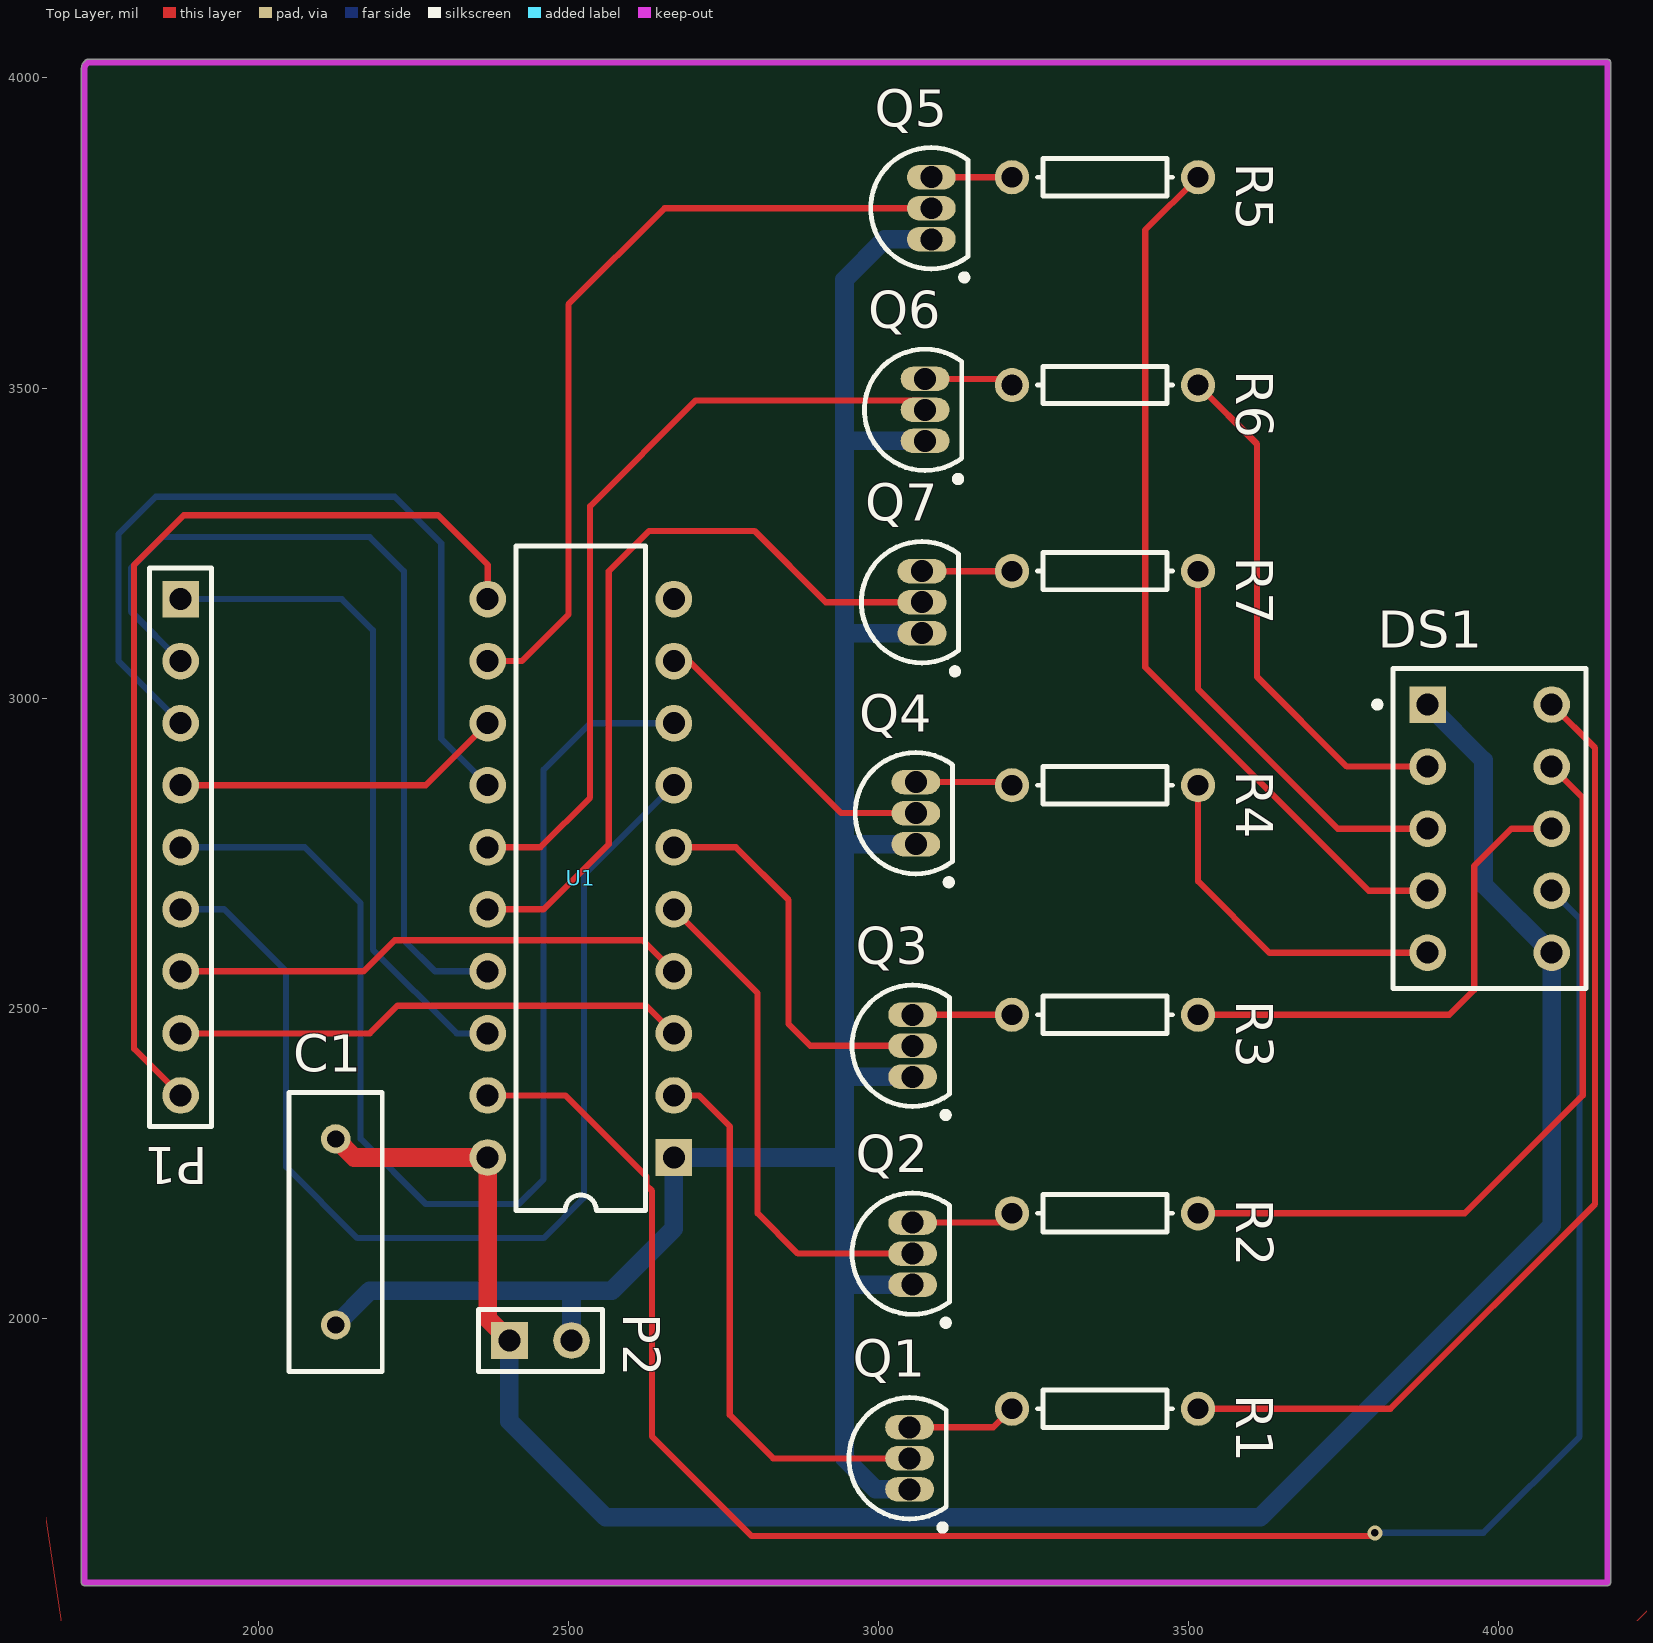
[diagram p0: Top Layer view]
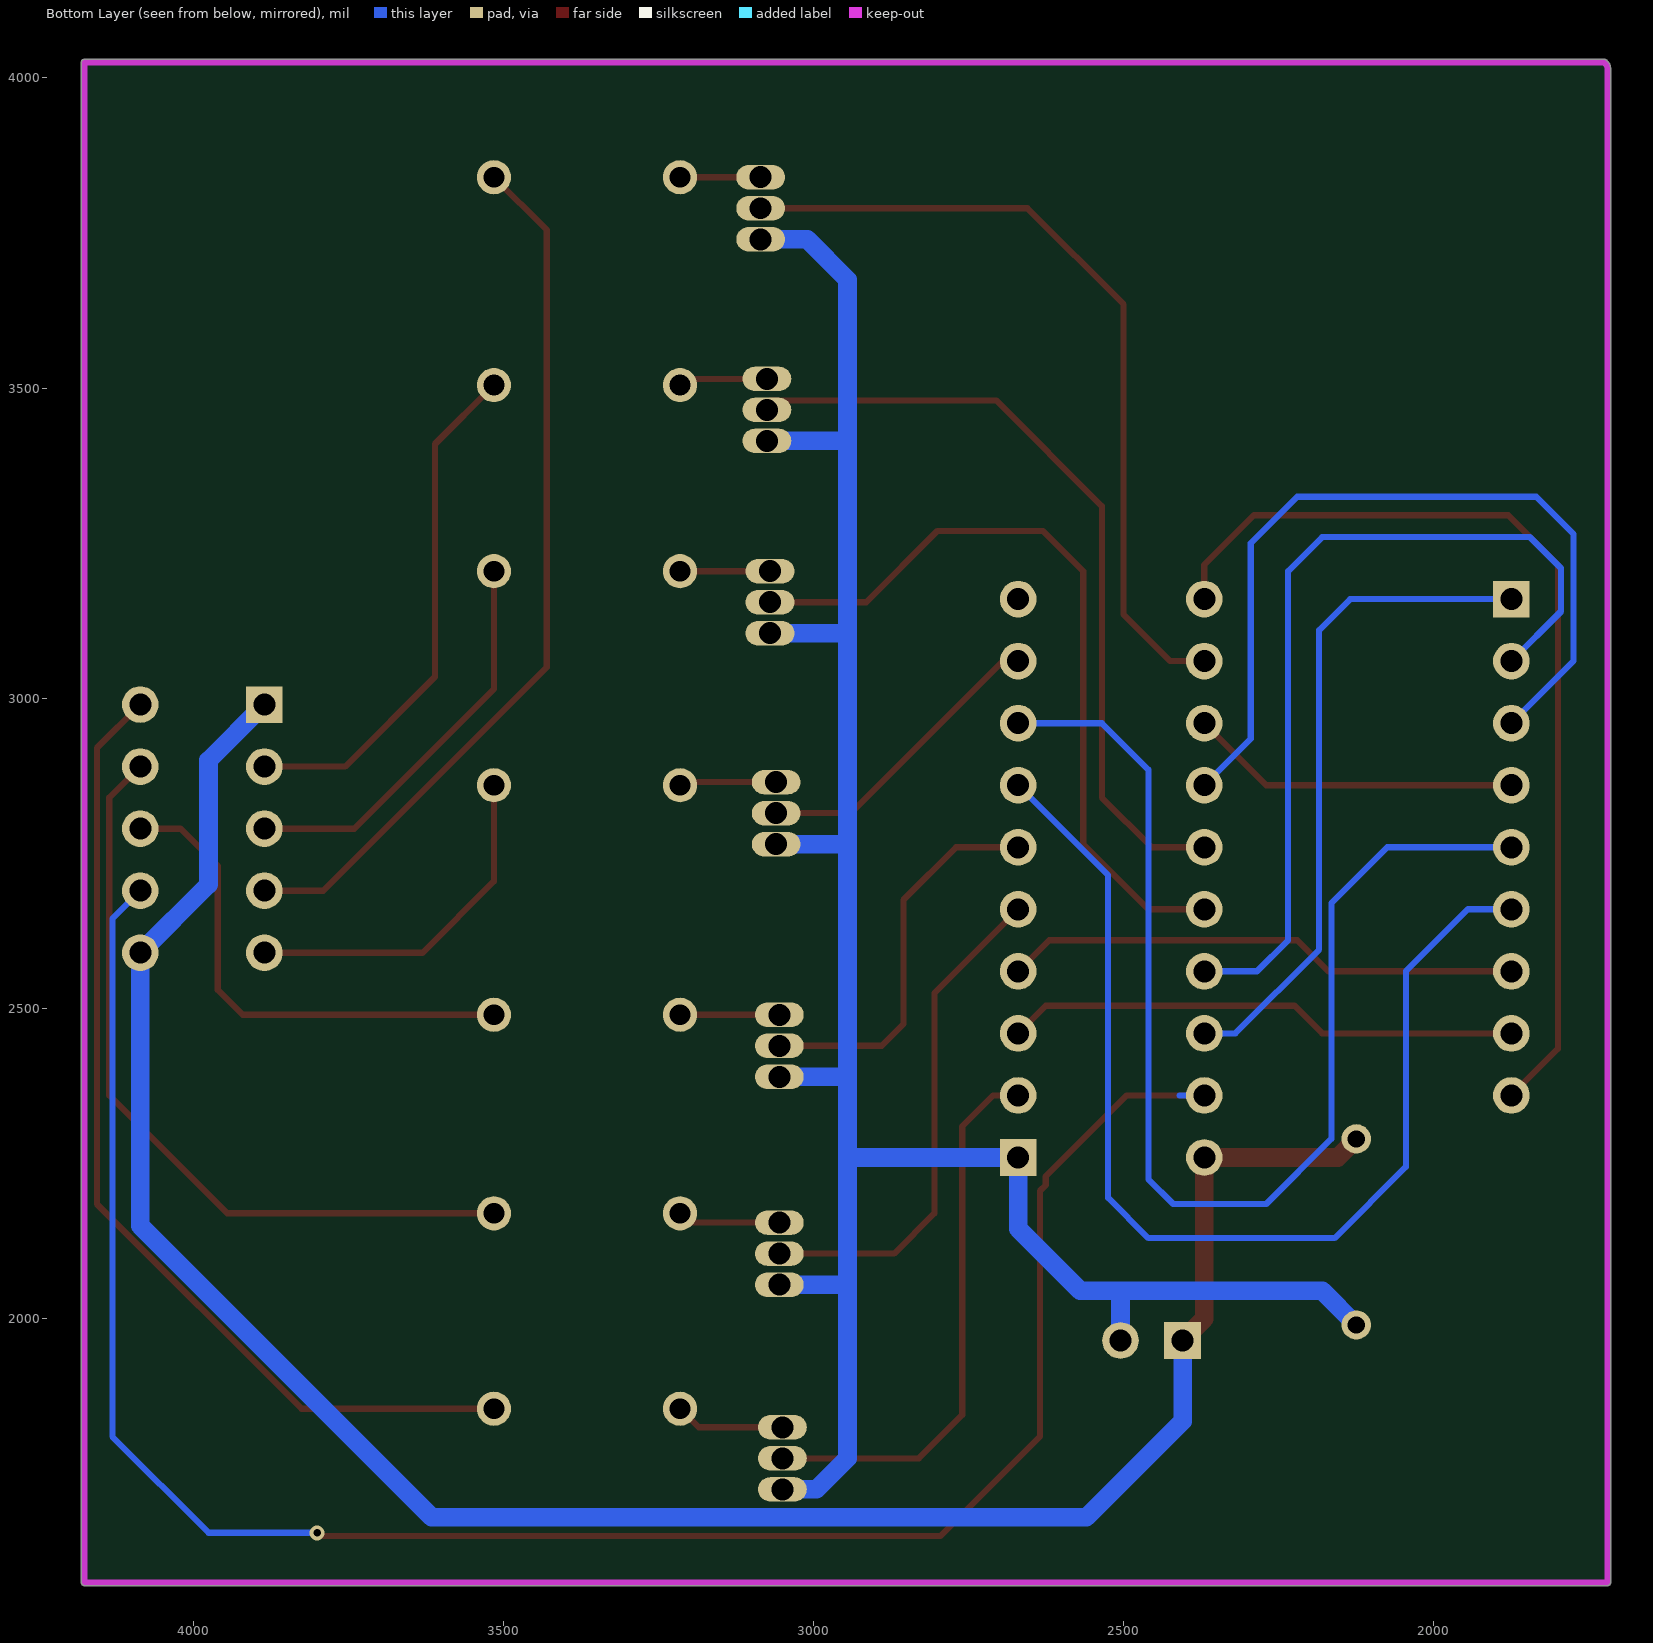
[diagram p1: Bottom Layer view, seen from below]
# Altium PCB MISC82807-2.PcbDoc
Units mil, origin at the board's own origin, x right, y up, seen from the top; angles counter-clockwise.
Board outline 2465.03 x 2460.03 mil, 2 copper layers (Top Layer, Bottom Layer); 19 components, 33 nets, 78 pads, 1 vias.

## Layer stack, top to bottom (the 12.6 mil dielectric is the usual default, probably not edited)
Top Solder: solder mask 0.4, Solder Resist, Dk 3.5
Top Layer: signal copper 1.4
Dielectric 1: dielectric 12.6, FR-4, Dk 4.8
Bottom Layer: signal copper 1.4
Bottom Solder: solder mask 0.4, Solder Resist, Dk 3.5

## Board outline
1714.98,1575 1714.98,4015 cw(c1732.07,4015) 1719.99,4027.08 1721.45,4028.55 1721.44,4028.53 cw(c1725,4025) 1725,4030.01 4175,4030.01 cw(c4175,4025) 4180.02,4025 4180.02,1575 cw(c4175,1575) 4175,1569.98 1720,1569.98 cw(c1720,1575)

## Design rules (kind name [scope] priority, off if disabled: settings)
AssemblyTestPointUsage [All] p0: scope1count=1 scope1_0_kind=Board scope1_0_value=Board scope2count=1 scope2_0_kind=Board scope2_0_value=Board commentlength=0
AssemblyTestpoint [All] p0: scope1count=1 scope1_0_kind=Board scope1_0_value=Board scope2count=1 scope2_0_kind=Board scope2_0_value=Board commentlength=0
Clearance [All] p0: scope1count=1 scope1_0_kind=Board scope1_0_value=Board scope2count=1 scope2_0_kind=Board scope2_0_value=Board commentlength=0 gap=10
Clearance [All] p1: gap=10
ComponentClearance [All] p0: scope1count=1 scope1_0_kind=Board scope1_0_value=Board scope2count=1 scope2_0_kind=Board scope2_0_value=Board commentlength=0 gap=10 collisioncheckmode=3
DiffPairsRouting [All] p0: scope1count=1 scope1_0_kind=Board scope1_0_value=Board scope2count=1 scope2_0_kind=Board scope2_0_value=Board commentlength=0
FabricationTestPointUsage [All] p0: scope1count=1 scope1_0_kind=Board scope1_0_value=Board scope2count=1 scope2_0_kind=Board scope2_0_value=Board commentlength=0 valid=0 allowmultiple=FALSE
FabricationTestpoint [All] p0: scope1count=1 scope1_0_kind=Board scope1_0_value=Board scope2count=1 scope2_0_kind=Board scope2_0_value=Board commentlength=0 side=3 testpointundercomponent=TRUE minsize=40 maxsize=100 preferedsize=60 minholesize=0 maxholesize=40 preferedholesize=32 testpointgrid=1
FanoutControl Fanout_Default [All] p0: scope1count=1 scope1_0_kind=Board scope1_0_value=Board scope2count=1 scope2_0_kind=Board scope2_0_value=Board commentlength=30 // Fanout_Default (Default Rule)
FanoutControl Fanout_Small [All] p0 off: scope1count=1 scope1_0_kind=Board scope1_0_value=Board scope2count=1 scope2_0_kind=Board scope2_0_value=Board commentlength=84 // Protel DXP Scope 1 Expression Was: (CompPinCount < 5)   Fanout_Small (Default Rule)
FanoutControl Fanout_SOIC [All] p0 off: scope1count=1 scope1_0_kind=Board scope1_0_value=Board scope2count=1 scope2_0_kind=Board scope2_0_value=Board commentlength=71 // Protel DXP Scope 1 Expression Was: IsSOIC   Fanout_SOIC (Default Rule)
FanoutControl Fanout_LCC [All] p0 off: scope1count=1 scope1_0_kind=Board scope1_0_value=Board scope2count=1 scope2_0_kind=Board scope2_0_value=Board commentlength=69 // Protel DXP Scope 1 Expression Was: IsLCC   Fanout_LCC (Default Rule)
FanoutControl Fanout_BGA [All] p0 off: scope1count=1 scope1_0_kind=Board scope1_0_value=Board scope2count=1 scope2_0_kind=Board scope2_0_value=Board commentlength=69 // Protel DXP Scope 1 Expression Was: IsBGA   Fanout_BGA (Default Rule)
Height [All] p0: scope1count=1 scope1_0_kind=Board scope1_0_value=Board scope2count=1 scope2_0_kind=Board scope2_0_value=Board commentlength=0
HoleSize [All] p0: scope1count=1 scope1_0_kind=Board scope1_0_value=Board scope2count=1 scope2_0_kind=Board scope2_0_value=Board commentlength=0 absolutevalues=TRUE maxlimit=100 minlimit=1 maxpercent=80.000 minpercent=20.000
HoleToHoleClearance [All] p0: scope1count=1 scope1_0_kind=Board scope1_0_value=Board scope2count=1 scope2_0_kind=Board scope2_0_value=Board commentlength=0
LayerPairs [All] p0: scope1count=1 scope1_0_kind=Board scope1_0_value=Board scope2count=1 scope2_0_kind=Board scope2_0_value=Board commentlength=0 enforce=TRUE
MinimumSolderMaskSliver [All] p0: scope1count=1 scope1_0_kind=Board scope1_0_value=Board scope2count=1 scope2_0_kind=Board scope2_0_value=Board commentlength=0
MinimumSolderMaskSliver [All] p1: minsoldermaskwidth=0
NetAntennae [All] p0: scope1count=1 scope1_0_kind=Board scope1_0_value=Board scope2count=1 scope2_0_kind=Board scope2_0_value=Board commentlength=0
PasteMaskExpansion [All] p0: scope1count=1 scope1_0_kind=Board scope1_0_value=Board scope2count=1 scope2_0_kind=Board scope2_0_value=Board commentlength=0 expansion=0
PlaneClearance [All] p0: scope1count=1 scope1_0_kind=Board scope1_0_value=Board scope2count=1 scope2_0_kind=Board scope2_0_value=Board commentlength=0 clearance=20
PlaneConnect [All] p0: scope1count=1 scope1_0_kind=Board scope1_0_value=Board scope2count=1 scope2_0_kind=Board scope2_0_value=Board commentlength=0 planeconnectstyle=Relief reliefexpansion=20 reliefentries=4 reliefconductorwidth=10 reliefairgap=10
PolygonConnect [All] p0: scope1count=1 scope1_0_kind=Board scope1_0_value=Board scope2count=1 scope2_0_kind=Board scope2_0_value=Board commentlength=0 connectstyle=Relief reliefconductorwidth=10 reliefentries=4 polygonreliefangle="90 Angle"
PolygonConnect [All] p1: connectstyle=Relief reliefconductorwidth=10 reliefentries=4 polygonreliefangle="90 Angle" airgapwidth=10
RoutingCorners [All] p0: scope1count=1 scope1_0_kind=Board scope1_0_value=Board scope2count=1 scope2_0_kind=Board scope2_0_value=Board commentlength=0 cornerstyle=45-Degree minsetback=100 maxsetback=100
RoutingLayers [All] p0: scope1count=1 scope1_0_kind=Board scope1_0_value=Board scope2count=1 scope2_0_kind=Board scope2_0_value=Board commentlength=0 top layer=Automatic bottom layer=Automatic
RoutingPriority [All] p0: scope1count=1 scope1_0_kind=Board scope1_0_value=Board scope2count=1 scope2_0_kind=Board scope2_0_value=Board commentlength=0
RoutingTopology [All] p0: scope1count=1 scope1_0_kind=Board scope1_0_value=Board scope2count=1 scope2_0_kind=Board scope2_0_value=Board commentlength=0 topology=Shortest
RoutingVias [All] p0: scope1count=1 scope1_0_kind=Board scope1_0_value=Board scope2count=1 scope2_0_kind=Board scope2_0_value=Board commentlength=0 holewidth=28 width=50 viastyle="Through Hole" minholewidth=28 minwidth=50 maxholewidth=28 maxwidth=50
RoutingVias [All] p1: holewidth=28 width=50 viastyle="Through Hole" minholewidth=28 minwidth=50 maxholewidth=28 maxwidth=50
ShortCircuit [All] p0: scope1count=1 scope1_0_kind=Board scope1_0_value=Board scope2count=1 scope2_0_kind=Board scope2_0_value=Board commentlength=0 allowed=FALSE
SilkToBoardRegionClearance [All] p0: scope1count=1 scope1_0_kind=Board scope1_0_value=Board scope2count=1 scope2_0_kind=Board scope2_0_value=Board commentlength=0
SilkToSilkClearance [All] p0: scope1count=1 scope1_0_kind=Board scope1_0_value=Board scope2count=1 scope2_0_kind=Board scope2_0_value=Board commentlength=0
SilkToSilkClearance [All] p1: silktosilkclearance=0
SilkToSolderMaskClearance [All] p0 off: scope1count=1 scope1_0_kind=Board scope1_0_value=Board scope2count=1 scope2_0_kind=Board scope2_0_value=Board commentlength=44 // Protel DXP Scope 1 Expression Was: IsPad
SilkToSolderMaskClearance [IsPad] p1: minsilkscreentomaskgap=0 clearancetoexposedcopper=TRUE
SolderMaskExpansion [All] p0: scope1count=1 scope1_0_kind=Board scope1_0_value=Board scope2count=1 scope2_0_kind=Board scope2_0_value=Board commentlength=0 expansion=4
SolderMaskExpansion [All] p1: expansion=4
UnRoutedNet [All] p0: scope1count=1 scope1_0_kind=Board scope1_0_value=Board scope2count=1 scope2_0_kind=Board scope2_0_value=Board commentlength=0
UnpouredPolygon [All] p0: scope1count=1 scope1_0_kind=Board scope1_0_value=Board scope2count=1 scope2_0_kind=Board scope2_0_value=Board commentlength=0
Width [All] p0: scope1count=1 scope1_0_kind=Board scope1_0_value=Board scope2count=1 scope2_0_kind=Board scope2_0_value=Board commentlength=0 maxlimit=30 minlimit=10 preferedwidth=10
Width [All] p1: maxlimit=30 minlimit=10 preferedwidth=10
27 further rules are at their usual default settings.

## Components (designator, comment, footprint, x,y, rotation, side; value= is the part's Value field where it differs from the comment)
C1 "Value" RAD-0.3 2125,2140 r90 top
DS1 "Dpy Red-CA" A 3985,2790 r0 top
P1 "Header 9" HDR1X9 1875,3160 r270 top
P2 "Header 2" HDR1X2 2405,1965 r0 top
Q1 "2N222A" TO-92A 3050,1775 r0 top
Q2 "2N222A" TO-92A 3055,2105 r0 top
Q3 "2N222A" TO-92A 3055,2440 r0 top
Q4 "2N222A" TO-92A 3060,2815 r0 top
Q5 "2N222A" TO-92A 3085,3790 r0 top
Q6 "2N222A" TO-92A 3075,3465 r0 top
Q7 "2N222A" TO-92A 3070,3155 r0 top
R1 "Value" AXIAL-0.3 3365,1855 r0 top
R2 "Value" AXIAL-0.3 3365,2170 r0 top
R3 "Value" AXIAL-0.3 3365,2490 r0 top
R4 "Value" AXIAL-0.3 3365,2860 r0 top
R5 "Value" AXIAL-0.3 3365,3840 r0 top
R6 "Value" AXIAL-0.3 3365,3505 r0 top
R7 "Value" AXIAL-0.3 3365,3205 r0 top
U1 "SN74LS373N" 738-03 2520,2710 r90 top

## Footprints (in the part's own frame and the unit in brackets; to place one, negate y for a bottom-side part, rotate by r counter-clockwise, add the part's x,y. Pads: shape width x height; smd on the part's side, far side on the other; paste and mask are expansions set on the pad)
738-03 [mm] "DIP; 20 Leads; Row Spacing 7.62 mm; Pitch 2.54 mm"
  rect 1.5x1.5 hole 0.9: 1(-11.43,-3.81)
  round 1.5 hole 0.9: 2(-8.89,-3.81) 3(-6.35,-3.81) 4(-3.81,-3.81) 5(-1.27,-3.81) 6(1.27,-3.81) 7(3.81,-3.81) 8(6.35,-3.81) 9(8.89,-3.81) 10(11.43,-3.81) 11(11.43,3.81) 12(8.89,3.81) 13(6.35,3.81) 14(3.81,3.81) 15(1.27,3.81) 16(-1.27,3.81) 17(-3.81,3.81) 18(-6.35,3.81) 19(-8.89,3.81) 20(-11.43,3.81)
  silkscreen extent -13.6,-2.65 13.6,2.65
A [mm] "LED, 7-Segment Display, 7.62 mm, RHD; 10 Leads; Row Space 5.08 mm; Pitch 2.54 mm"
  rect 1.5x1.5 hole 0.9: 1(-2.54,5.08)
  round 1.5 hole 0.9: 2(-2.54,2.54) 3(-2.54,0) 4(-2.54,-2.54) 5(-2.54,-5.08) 6(2.54,-5.08) 7(2.54,-2.54) 8(2.54,0) 9(2.54,2.54) 10(2.54,5.08)
  silkscreen extent -4.72,-6.55 3.95,6.55
AXIAL-0.3 [mm] "Axial Device, Thru-Hole; 2 Leads; 0.3 in Pin Spacing"
  round 1.4 hole 0.85: 1(-3.81,0) 2(3.81,0)
  silkscreen extent -2.77,-0.76 2.77,0.76
HDR1X2 [mm] "Connector; Header; 2 Position"
  rect 1.5x1.5 hole 0.9: 1(0,0)
  round 1.5 hole 0.9: 2(2.54,0)
  silkscreen extent -1.27,-1.27 3.81,1.27
HDR1X9 [mm] "Connector; Header; 9 Position"
  rect 1.5x1.5 hole 0.9: 1(0,0)
  round 1.5 hole 0.9: 2(2.54,0) 3(5.08,0) 4(7.62,0) 5(10.16,0) 6(12.7,0) 7(15.24,0) 8(17.78,0) 9(20.32,0)
  silkscreen extent -1.27,-1.27 21.59,1.27
RAD-0.3 [mm] "Radial Cap, Thru-Hole; 2 Leads; 0.3 in Pin Spacing"
  round 1.2 hole 0.7: 1(-3.81,0) 2(3.81,0)
  silkscreen extent -5.71,-1.91 5.71,1.91
TO-92A [mm] "TO, Flat Index; 3 In-Line, Axial Leads; Body Dia. 4.5mm; Leads 0.51 x 0.48 mm (max)"
  oval 2x1 hole 0.9: 1(0,-1.27) 2(0,0) 3(0,1.27)
  silkscreen extent -2.48,-2.95 1.5,2.48

## Part data
C1: library part Cap, "Capacitor"
DS1: "7.62 mm Black Surface HER 7-Segment Display: CA, RH DP"
P1: "Header, 9-Pin"
P2: "Header, 2-Pin"
Q1 Q2 Q3 Q4 Q5 Q6 Q7: library part 2N3904, "NPN General Purpose Amplifier"
R1 R2 R3 R4 R5 R6 R7: library part Res1, "Resistor"
U1: "Octal Transparent Latch with 3-State Outputs"

## Via types
v1: diameter 24, hole 12, Top Layer to Bottom Layer, 1 vias

## Nets (pads, with @x,y where several pads share a name; then routed paths per layer and width w, separated by ;. In a path a pad name is that pad's centre, name@x,y a point inside that pad or via, vN(x,y) a via of type N, cw(c..) or ccw(c..) an arc to the next point about the centre after c; other vN are vias at no path point)
DATA0: P1.8 U1.3 | length 831.9
  Top Layer w10: P1.8 2180,2460 2224.53,2504.53 2625.47,2504.53 U1.3
DATA1: P1.7 U1.4 | length 836.4
  Top Layer w10: P1.7 2170,2560 2220,2610 2620,2610 U1.4
DATA2: P1.6 U1.7 | length 1806
  Bottom Layer w10: P1.6 1945,2660 2045,2560 2045,2245 2160,2130 2460,2130 2525,2195 2525,2715 U1.7
DATA3: P1.5 U1.8 | length 1963.4
  Bottom Layer w10: P1.5 2075,2760 2165,2670 2165,2290 2270,2185 2420,2185 2460,2225 2460,2885 2535,2960 U1.8
DATA4: P1.4 U1.13 | length 536.4
  Top Layer w10: P1.4 2270,2860 U1.13
DATA5: P1.3 U1.14 | length 1343.4
  Bottom Layer w10: P1.3 1775,3060 1775,3265 1835,3325 2220,3325 2295,3250 2295,2935 U1.14
DATA6: P1.2 U1.17 | length 1417.3
  Bottom Layer w10: P1.2 1795,3140 1795,3210 1845,3260 2180,3260 2235,3205 2235,2610 2285,2560 U1.17
DATA7: P1.1 U1.18 | length 1086.6
  Bottom Layer w10: P1.1 2135,3160 2185,3110 2185,2595 2320,2460 U1.18
GND: C1.1 P2.2 Q1.1 Q2.1 Q3.1 Q4.1 Q5.1 Q6.1 Q7.1 U1.1 | length 3866
  Bottom Layer w30: C1.1 2180,2045 2505,2045 ; P2.2 2505,2045 ; Q1.1 2995,1725 2945,1775 2945,2055 ; Q2.1 2945,2055 ; Q3.1 2950,2390 2945,2395 ; Q4.1 2945,2765 ; Q7.1 2945,3105 ; Q6.1 2945,3415 ; Q5.1 3010,3740 2945,3675 2945,3415 ; 2505,2045 2570,2045 2670,2145 U1.1 2940,2260 2945,2255 ; 2945,2055 2945,2255 ; 2945,2255 2945,2395 ; 2945,2395 2945,2765 ; 2945,2765 2945,3105 ; 2945,3105 2945,3415
NetDS1_2: DS1.2 R6.2 | length 844.4
  Top Layer w10: R6.2 3610,3410 3610,3035 3755,2890 DS1.2
NetDS1_3: DS1.3 R7.2 | length 653.2
  Top Layer w10: R7.2 3515,3015 3740,2790 DS1.3
NetDS1_4: DS1.4 R5.2 | length 1429.3
  Top Layer w10: R5.2 3430,3755 3430,3050 3790,2690 DS1.4
NetDS1_5: DS1.5 R4.2 | length 572.6
  Top Layer w10: R4.2 3515,2705 3630,2590 DS1.5
NetDS1_7: DS1.7 U1.19 | length 3302.1
  Top Layer w10: U1.19 2495,2360 2625.47,2229.53 2625.47,2215.47 2635,2205.95 2635,1810 2795,1650 v1@3805,1650
  Bottom Layer w10: U1.19 2410,2360 ; v1(3800,1655) 3975,1655 4130,1810 4130,2645 DS1.7
NetDS1_8: DS1.8 R3.2 | length 811.4
  Top Layer w10: R3.2 3920,2490 3960,2530 3960,2730 4020,2790 DS1.8
NetDS1_9: DS1.9 R2.2 | length 1249.4
  Top Layer w10: R2.2 3945,2170 4135,2360 4135,2840 DS1.9
NetDS1_10: DS1.10 R1.2 | length 1610.7
  Top Layer w10: R1.2 3825,1855 4155,2185 4155,2920 DS1.10
NetP1_9: P1.9 U1.11 | length 1577.3
  Top Layer w10: P1.9 1800,2435 1800,3215 1880,3295 2290,3295 2370,3215 U1.11
NetQ1_2: Q1.2 U1.2 | length 894.7
  Top Layer w10: U1.2 2710,2360 2760,2310 2760,1845 2830,1775 Q1.2
NetQ1_3: Q1.3 R1.1 | length 177.4
  Top Layer w10: Q1.3 3185,1825 R1.1
NetQ2_2: Q2.2 U1.5 | length 822.8
  Top Layer w10: U1.5 2805,2525 2805,2170 2870,2105 Q2.2
NetQ2_3: Q2.3 R2.1 | length 166.2
  Top Layer w10: Q2.3 3200,2155 R2.1
NetQ3_2: Q3.2 U1.6 | length 634.7
  Top Layer w10: U1.6 2770,2760 2855,2675 2855,2475 2890,2440 Q3.2
NetQ3_3: Q3.3 R3.1 | length 160
  Top Layer w10: Q3.3 R3.1
NetQ4_2: Q4.2 U1.9 | length 491.5
  Top Layer w10: U1.9 2695,3060 2940,2815 Q4.2
NetQ4_3: Q4.3 R4.1 | length 157.1
  Top Layer w10: Q4.3 3210,2865 R4.1
NetQ5_2: Q5.2 U1.12 | length 1310.3
  Top Layer w10: U1.12 2425,3060 2500,3135 2500,3635 2655,3790 Q5.2
NetQ5_3: Q5.3 R5.1 | length 130
  Top Layer w10: Q5.3 R5.1
NetQ6_2: Q6.2 U1.15 | length 1273.7
  Top Layer w10: U1.15 2455,2760 2535,2840 2535,3310 2705.32,3480.32 Q6.2@3070,3480.32
NetQ6_3: Q6.3 R6.1 | length 144.1
  Top Layer w10: Q6.3 3205,3515 R6.1
NetQ7_2: Q7.2 U1.16 | length 1258.1
  Top Layer w10: U1.16 2460,2660 2565,2765 2565,3205 2630,3270 2800,3270 2915,3155 Q7.2
NetQ7_3: Q7.3 R7.1 | length 145
  Top Layer w10: Q7.3 R7.1
VCC: C1.2 DS1.1 DS1.6 P2.1 U1.20 | length 3558.7
  Top Layer w30: C1.2 2155,2260 U1.20 2370,2000 P2.1
  Bottom Layer w30: P2.1 2405,1835 2560,1680 3615,1680 4085,2150 DS1.6 3975,2700 3975,2900 DS1.1
pads on no net: U1.10

## Polygon pours and split planes (outlines as drawn)
GND on Bottom Layer "D" (solid, remove dead copper, pour order 0): 1315,4440 4550,4440 4620,4370 4315,4065 4315,1400 1435,1400 1410,1425
GND on Top Layer "D" (solid, remove dead copper, pour order 2): 1275,4245 1350,4320 4735,4320 4735,2025 4015,1305 4010,1300 1715,1300

## Keep-outs
Keep-Out Layer:
  lines w10: 3035,4025 4175,4025 4175,1575 1720,1575 1720,1670 1720,1680 1720,1850 1720,4015 cw(c1732.07,4015) 1723.54,4023.54 1725,4025 3050,4025